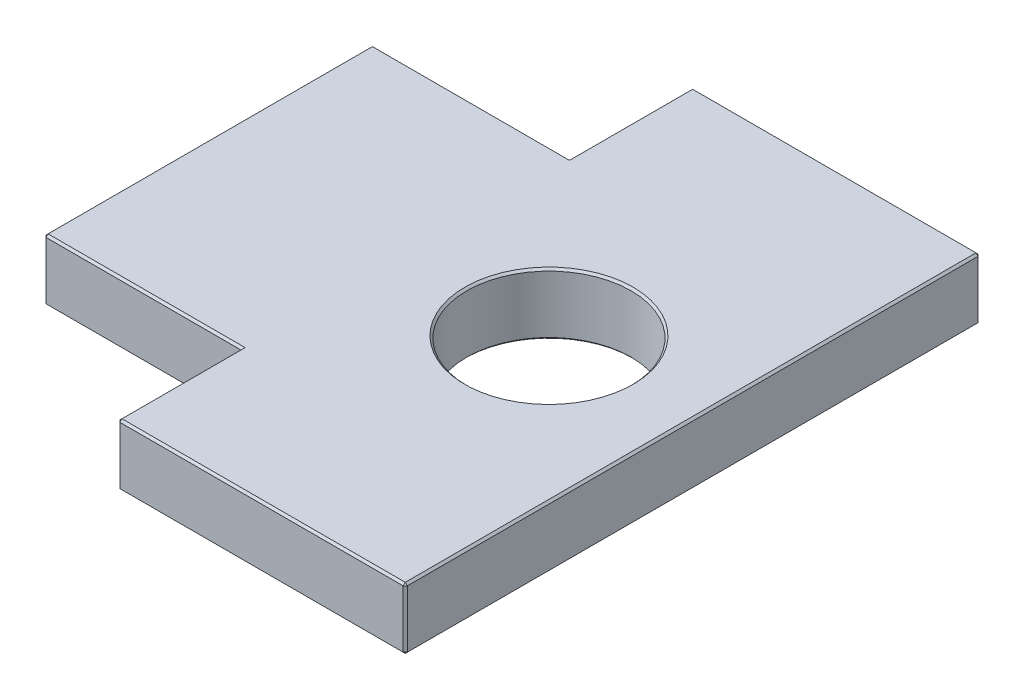
SolidWorks part; units mm, degrees
material "合金钢"
ref_plane "前视基准面" through (0, 0, 0) normal (0, 0, 1) x (1, 0, 0)
ref_plane "上视基准面" through (0, 0, 0) normal (0, 1, 0) x (1, 0, 0)
ref_plane "右视基准面" through (0, 0, 0) normal (1, 0, 0) x (0, 0, -1)
sketch "草图1" plane through (0, 0, 0) normal (0, 1, 0) x (1, 0, 0)
  line L0 (0, 70) -> (0, -70)
  line L1 (0, -70) -> (-70, -70)
  line L2 (-70, -70) -> (-70, -40)
  line L3 (-70, -40) -> (-118, -40)
  line L4 (-118, -40) -> (-118, 40)
  line L5 (-118, 40) -> (-70, 40)
  line L6 (-70, 40) -> (-70, 70)
  line L7 (-70, 70) -> (0, 70)
  circle A0 centre (-35, 0) radius 20
  point P4 (0, 0)
  point P12 (-118, 0)
  dimension "D5" = 40
  dimension "D6" = 15
  dimension "D1" = 140
  dimension "D2" = 80
  dimension "D3" = 48
  dimension "D4" = 70
extrude "凸台-拉伸1" add sketch "草图1" along normal blind 15
chamfer "倒角1" distance 0.5 angle 45 24 edges at (0, 7.5, -70) (0, 7.5, 70) (-70, 7.5, 70) (-118, 7.5, 40) (-70, 7.5, -70) (-118, 7.5, -40) (-35, 0, 20) (-70, 15, 55) (-94, 15, 40) (-118, 15, 0) (-94, 15, -40) (-70, 15, -55) (-35, 15, 70) (0, 15, 0) (-35, 15, -70) (-70, 0, 55) (-94, 0, 40) (-118, 0, 0) (-94, 0, -40) (-70, 0, -55) (-35, 0, -70) (0, 0, 0) (-35, 0, 70) (-35, 15, 20)
